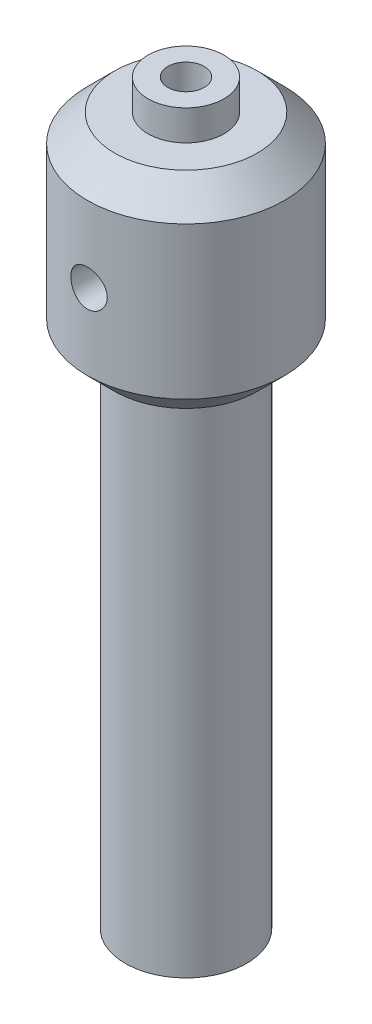
SolidWorks part; units mm, degrees
material "Copper"
ref_plane "Front Plane" through (0, 0, 0) normal (0, 0, 1) x (1, 0, 0)
ref_plane "Top Plane" through (0, 0, 0) normal (0, 1, 0) x (1, 0, 0)
ref_plane "Right Plane" through (0, 0, 0) normal (1, 0, 0) x (0, 0, -1)
sketch "Sketch1" plane through (0, 0, 0) normal (0, 0, 1) x (1, 0, 0)
  line L0 (0, 51.625) -> (12.5, 51.625)
  line L1 (12.5, 51.625) -> (12.5, 41.625)
  line L2 (0, 41.625) -> (23.5, 41.625)
  line L3 (23.5, 41.625) -> (32.5, 32.625)
  line L4 (32.5, 32.625) -> (0, 32.625)
  line L5 (0, 32.625) -> (0, 41.625)
  line L6 (0, 41.625) -> (0, 51.625)
  line L7 (0, 32.625) -> (0, -17.375)
  line L8 (0, -17.375) -> (32.5, -17.375)
  line L9 (32.5, -17.375) -> (32.5, 32.625)
  line L10 (0, -17.375) -> (0, -26.375)
  line L11 (0, -26.375) -> (23.5, -26.375)
  line L12 (23.5, -26.375) -> (32.5, -17.375)
  line L13 (0, -26.375) -> (0, -191.375)
  line L14 (0, -191.375) -> (20, -191.375)
  line L15 (20, -191.375) -> (20, -26.375)
  dimension "D1" = 10
  dimension "D2" = 9
  dimension "D3" = 12.5
  dimension "D4" = 165
  dimension "D6" = 32.5
  dimension "D7" = 9
  dimension "D8" = 45
  dimension "D9" = 45
  dimension "D10" = 20
revolve "Revolve7" add sketch "Sketch1" angle 360 about L13
sketch "Sketch5" plane through (0, 0, 0) normal (0, 0, 1) x (1, 0, 0)
  line L0 (0, 51.625) -> (0, 24.625)
  line L1 (12.5, 51.625) -> (-12.5, 51.625) construction
  line L2 (0, 51.625) -> (6, 51.625)
  line L3 (6, 51.625) -> (6, 24.625)
  line L4 (0, 24.625) -> (0, 21.625)
  line L5 (0, 21.625) -> (6, 24.625)
  dimension "D2" = 3
  dimension "D3" = 27
revolve "Cut-Revolve1" cut sketch "Sketch5" angle 360 about L0
sketch "Sketch6" plane through (0, 0, 0) normal (0, 0, 1) x (1, 0, 0)
  line L0 (0, 32.625) -> (0, 7.625) construction
  line L1 (-32.5, 32.625) -> (32.5, 32.625) construction
  circle A0 centre (0, 7.625) radius 6
  dimension "D2" = 12
  dimension "D1" = 25
extrude "Cut-Extrude1" cut sketch "Sketch6" against normal mid plane 160 contours A0
